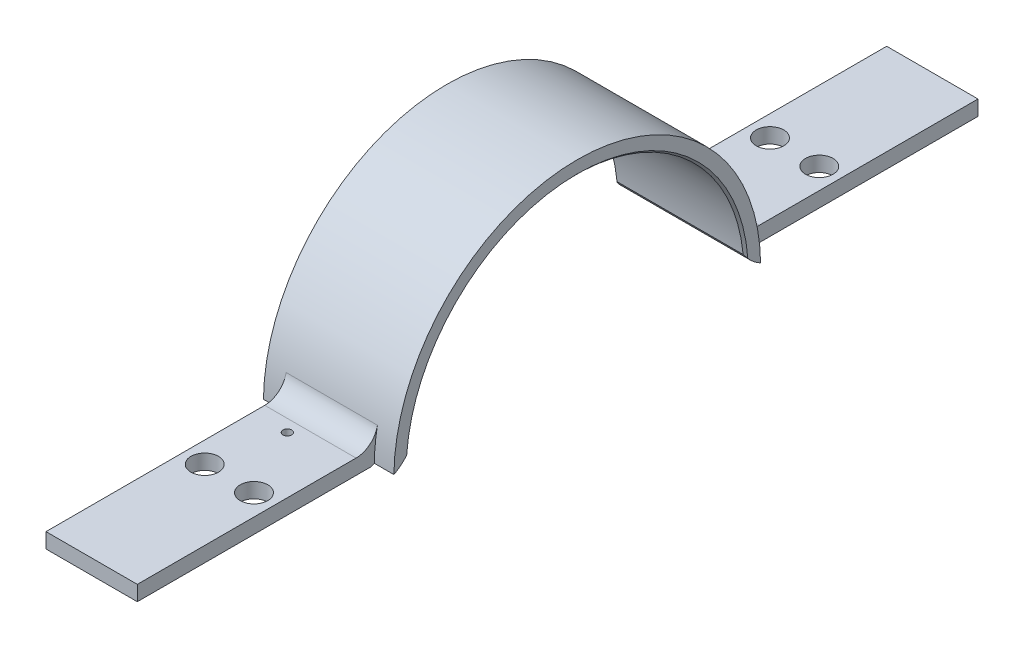
SolidWorks part; units mm, degrees
material "Q345B"
ref_plane "Front Plane" through (0, 0, 0) normal (0, 0, 1) x (1, 0, 0)
ref_plane "Top Plane" through (0, 0, 0) normal (0, 1, 0) x (1, 0, 0)
ref_plane "Right Plane" through (0, 0, 0) normal (1, 0, 0) x (0, 0, -1)
sketch "Sketch1" plane through (0, 0, 0) normal (1, 0, 0) x (0, 0, -1)
  line L0 (0, 30.477) -> (0, -16.0366) construction
  line L1 (-26.5083, 0) -> (25.5163, 0) construction
  line L2 (-580, 22) -> (-252.0417, 22)
  line L3 (252.0417, 22) -> (580, 22)
  line L4 (-580, -3) -> (-227.9803, -3)
  line L5 (227.9803, -3) -> (580, -3)
  line L6 (-580, 22) -> (-580, -3)
  line L7 (580, 22) -> (580, -3)
  arc A1 (227.9803, -3) -> (-227.9803, -3) centre (0, 0) ccw
  arc A3 (252.0417, 22) -> (-252.0417, 22) centre (0, 0) ccw
  dimension "D1" = 580
  dimension "D3" = 253
  dimension "D2" = 580
  dimension "D4" = 22
  dimension "D5" = 25
extrude "Boss-Extrude1" add sketch "Sketch1" along normal mid plane 180
fillet "Fillet1" radius 30 2 edges at (0, 22, -252.0417) (0, 22, 252.0417)
fillet "Fillet2" radius 55 2 edges at (0, -3, 227.9803) (0, -3, -227.9803)
sketch "Sketch2" plane through (0, 0, 0) normal (1, 0, 0) x (0, 0, -1)
  circle A0 centre (0, 0) radius 233
  dimension "D1" = 466
extrude "Cut-Extrude1" cut sketch "Sketch2" against normal through all both and the other way through all
sketch "Sketch3" plane through (0, 0, 0) normal (1, 0, 0) x (0, 0, -1)
  line L1 (-610, 1.2) -> (610, 1.2)
  line L2 (-610, 1.2) -> (-610, -20)
  line L3 (-610, -20) -> (610, -20)
  line L4 (610, 1.2) -> (610, -20)
  dimension "D1" = 610
  dimension "D2" = 610
  dimension "D3" = 1.2
  dimension "D4" = 20
extrude "Cut-Extrude2" cut sketch "Sketch3" against normal through all both and the other way through all
sketch "Sketch4" plane through (90, 0, 0) normal (1, 0, 0) x (0, 0, -1)
  line L1 (-598.0101, 50) -> (-248.0101, 50)
  line L2 (-598.0101, 50) -> (-598.0101, -20)
  line L3 (-598.0101, -20) -> (-252.2082, -20)
  arc A0 (248.6924, 46.4876) -> (-248.6924, 46.4876) centre (0, 0) ccw construction
  arc A5 (-248.0101, 50) -> (-252.2082, -20) centre (0, 0) ccw
  dimension "D1" = 50
  dimension "D2" = 20
  dimension "D5" = 350
extrude "Cut-Extrude3" cut sketch "Sketch4" against normal blind 27
mirror "Mirror1" about plane through (0, 0, 0) normal (0, 0, 1) of "Cut-Extrude3"
mirror "Mirror2" about plane through (0, 0, 0) normal (1, 0, 0) of "Mirror1", "Cut-Extrude3"
sketch "Sketch5" plane through (0, 0, 0) normal (0, 1, 0) x (1, 0, 0)
  line L0 (34, 668.832) -> (34, -639.6333) construction
  line L1 (-190.7038, 0) -> (185.229, 0) construction
  line L2 (0, 652.4077) -> (0, -656.0576) construction
  line L3 (-34, 668.832) -> (-34, -639.6333) construction
  circle A0 centre (34, -390) radius 19
  circle A1 centre (34, 390) radius 19
  circle A2 centre (-34, -390) radius 19
  circle A3 centre (-34, 390) radius 19
  circle A4 centre (-15, -295) radius 6
  circle A5 centre (15, 295) radius 6
  dimension "D1" = 390
  dimension "D2" = 38
  dimension "D4" = 12
  dimension "D3" = 68
  dimension "D5" = 15
  dimension "D6" = 95
  dimension "D7" = 95
  dimension "D8" = 15
extrude "Cut-Extrude4" cut sketch "Sketch5" against normal through all and the other way through all
chamfer "Chamfer1" distance 3 angle 45 2 edges at (-90, 233, 0) (90, 233, 0)
